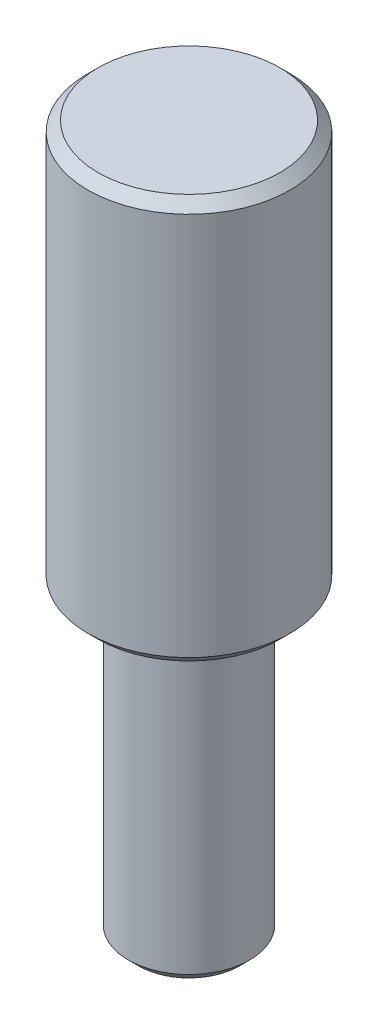
SolidWorks part; units mm, degrees
ref_plane "Front Plane" through (0, 0, 0) normal (0, 0, 1) x (1, 0, 0)
ref_plane "Top Plane" through (0, 0, 0) normal (0, 1, 0) x (1, 0, 0)
ref_plane "Right Plane" through (0, 0, 0) normal (1, 0, 0) x (0, 0, -1)
sketch "Sketch1" plane through (0, 0, 0) normal (0, 1, 0) x (1, 0, 0)
  circle A0 centre (0, 0) radius 5
  dimension "D1" = 10
extrude "Boss-Extrude1" add sketch "Sketch1" along normal blind 20
sketch "Sketch2" plane through (0, 0, 0) normal (0, -1, 0) x (1, 0, 0)
  circle A0 centre (0, 0) radius 3
  dimension "D1" = 6
extrude "Boss-Extrude2" add sketch "Sketch2" along normal blind 15
cosmetic thread "Cosmetic Thread1" parameters "D2"=5.16
chamfer "Chamfer1" distance 0.5 angle 45 3 edges at (0, 20, 5) (0, 0, 5) (0, -15, -3)
